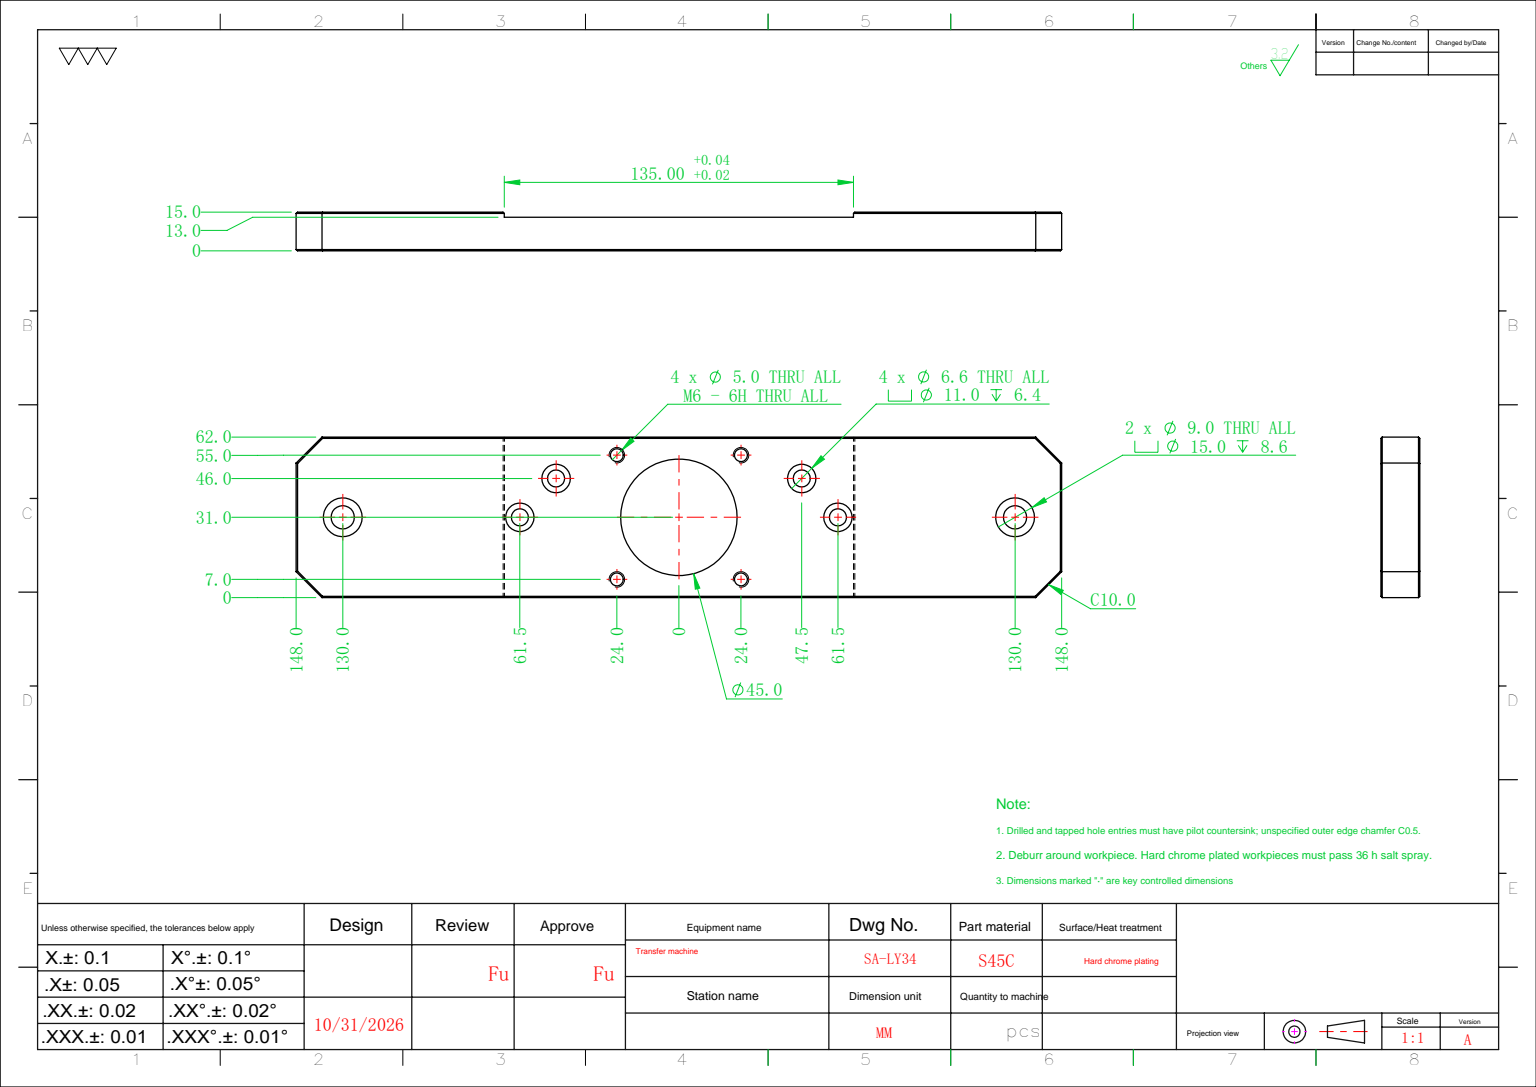
SolidWorks part; units mm, degrees
material "S45C"
ref_plane "前视基准面" through (0, 0, 0) normal (0, 0, 1) x (1, 0, 0)
ref_plane "上视基准面" through (0, 0, 0) normal (0, 1, 0) x (1, 0, 0)
ref_plane "右视基准面" through (0, 0, 0) normal (1, 0, 0) x (0, 0, -1)
sketch "草图1" plane through (0, 0, 0) normal (0, 0, 1) x (1, 0, 0)
  line L1 (-148, -31) -> (148, -31)
  line L2 (-148, -31) -> (-148, 31)
  line L3 (-148, 31) -> (148, 31)
  line L4 (148, -31) -> (148, 31)
  line L5 (-148, -31) -> (148, 31) construction
  line L6 (-148, 31) -> (148, -31) construction
  point P0 (0, 0)
  dimension "D1" = 296
  dimension "D2" = 62
extrude "凸台-拉伸1" add sketch "草图1" along normal blind 15
chamfer "倒角1" distance 10 angle 45 4 edges at (148, 31, 7.5) (148, -31, 7.5) (-148, 31, 7.5) (-148, -31, 7.5)
sketch "草图3" plane through (0, 0, 0) normal (0, 0, -1) x (-1, 0, 0)
  circle A0 centre (0, 0) radius 22.5
  dimension "D1" = 45
extrude "切除-拉伸2" cut sketch "草图3" against normal through all
hole_wizard "M6 螺纹孔1" positions "草图4" profile "草图5" tap size "M6" standard "ISO" end condition through all
sketch "草图4" plane through (0, 0, 15) normal (0, 0, 1) x (1, 0, 0)
  line L0 (0, 0) -> (49.1231, 0) construction
  line L2 (0, 0) -> (0, -57.1761) construction
  point P0 (-24, 24)
  point P3 (24, 24)
  point P6 (24, -24)
  point P9 (-24, -24)
  dimension "D1" = 48
  dimension "D2" = 48
sketch "草图5" plane through (-24, 24, 15) normal (1, 0, 0) x (0, -1, 0)
  line L0 (0, 0) -> (0, 15)
  line L1 (0, 15) -> (2.5, 15)
  line L2 (2.5, 15) -> (2.5, 0)
  line L5 (2.5, 0) -> (0, 0)
  line L11 (0, -6.35) -> (0, 107.95) construction
  dimension "通孔螺纹孔钻头直径" = 5
  dimension "通孔螺纹孔钻头深度" = 15
cosmetic thread "孔螺蚊线1" parameters "D2"=6
cosmetic thread "孔螺蚊线2" parameters "D2"=6
cosmetic thread "孔螺蚊线3" parameters "D2"=6
cosmetic thread "孔螺蚊线4" parameters "D2"=6
sketch "草图6" plane through (0, -31, 0) normal (0, -1, 0) x (1, 0, 0)
  line L0 (-138, 0) -> (138, 0) construction
  line L1 (-67.5, 0) -> (67.5, 0)
  line L2 (-67.5, 0) -> (-67.5, 2)
  line L3 (-67.5, 2) -> (67.5, 2)
  line L4 (67.5, 0) -> (67.5, 2)
  line L5 (0, 0) -> (0, 12.955) construction
  dimension "D1" = 135
  dimension "D2" = 2
extrude "切除-拉伸3" cut sketch "草图6" against normal through all
hole_wizard "M6 六角凹头螺钉的柱形沉头孔1" positions "草图8" profile "草图9" counterbore size "M6" standard "ISO" end condition through all
sketch "草图8" plane through (0, 0, 15) normal (0, 0, 1) x (1, 0, 0)
  line L0 (0, 0) -> (0, 46.9151) construction
  point P0 (-47.5, 15)
  point P3 (-61.5, 0)
  point P6 (47.5, 15)
  point P9 (61.5, 0)
  dimension "D1" = 123
  dimension "D2" = 95
  dimension "D3" = 15
  dimension "D4" = 15
sketch "草图9" plane through (-47.5, 15, 15) normal (1, 0, 0) x (0, -1, 0)
  line L0 (0, 0) -> (0, 15)
  line L1 (0, 15) -> (3.3, 15)
  line L3 (3.3, 15) -> (3.3, 6.4)
  line L4 (3.3, 6.4) -> (5.5, 6.4)
  line L5 (5.5, 6.4) -> (5.5, 0)
  line L7 (5.5, 0) -> (0, 0)
  line L11 (0, -6.35) -> (0, 107.95) construction
  dimension "通孔孔直径" = 6.6
  dimension "通孔孔深度" = 15
  dimension "柱形沉头孔直径" = 11
  dimension "柱形沉头孔深度" = 6.4
hole_wizard "M8 六角凹头螺钉的柱形沉头孔1" positions "草图13" profile "草图14" counterbore size "M8" standard "ISO" end condition through all
sketch "草图13" plane through (0, 0, 15) normal (0, 0, -1) x (-1, 0, 0)
  line L0 (-130, 0) -> (130, 0) construction
  line L2 (0, 0) -> (0, 31) construction
  line L3 (-67.5, 31) -> (67.5, 31) construction
  line L5 (130, 0) -> (148, 0) construction
  line L6 (148, 21) -> (148, -21) construction
  point P0 (130, 0)
  point P3 (-130, 0)
  dimension "D1" = 260
sketch "草图14" plane through (-130, 0, 15) normal (1, 0, 0) x (0, -1, 0)
  line L0 (0, 0) -> (0, 15)
  line L1 (0, 15) -> (4.5, 15)
  line L3 (4.5, 15) -> (4.5, 8.6)
  line L4 (4.5, 8.6) -> (7.5, 8.6)
  line L5 (7.5, 8.6) -> (7.5, 0)
  line L7 (7.5, 0) -> (0, 0)
  line L11 (0, -6.35) -> (0, 107.95) construction
  dimension "通孔孔直径" = 9
  dimension "通孔孔深度" = 15
  dimension "柱形沉头孔直径" = 15
  dimension "柱形沉头孔深度" = 8.6
chamfer "倒角2" distance 0.5 angle 45 20 edges at (102.75, -31, 0) (143, -26, 0) (148, 0, 0) (143, 26, 0) (102.75, 31, 0) (67.5, 0, 0) (-102.75, 31, 0) (-143, 26, 0) (-148, 0, 0) (-143, -26, 0) (-102.75, -31, 0) (-67.5, 0, 0) (143, -26, 15) (0, -31, 15) (-143, -26, 15) (-148, 0, 15) (-143, 26, 15) (0, 31, 15) (143, 26, 15) (148, 0, 15)
